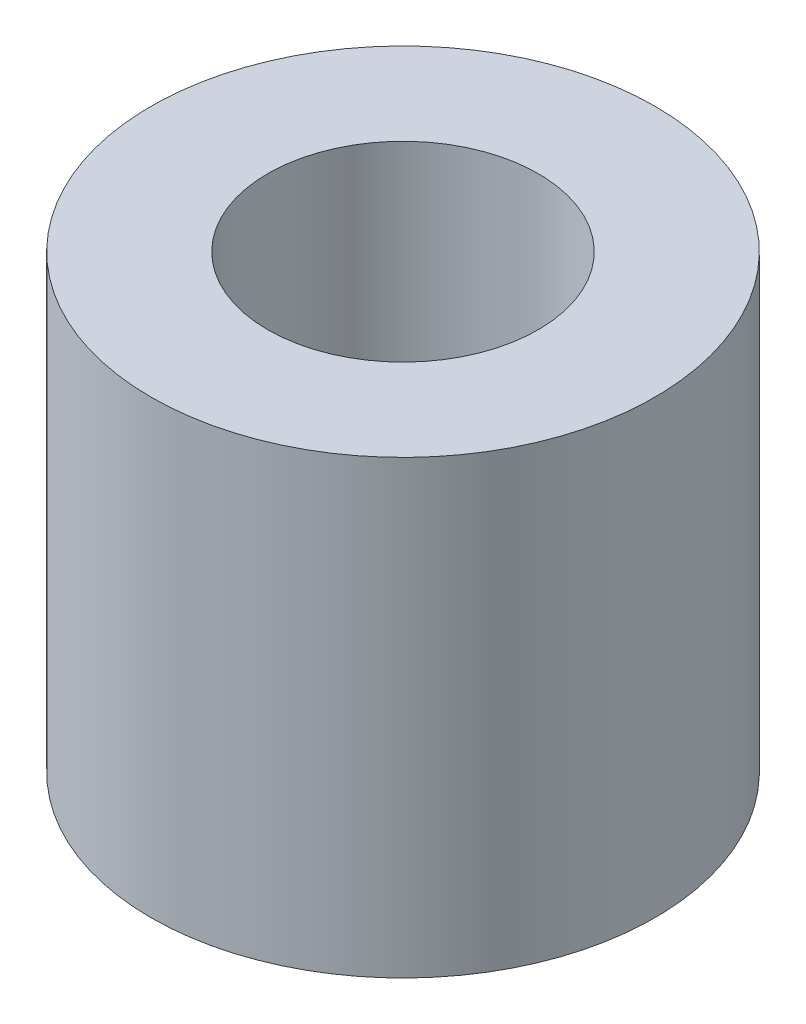
SolidWorks part; units mm, degrees
material "SS400P"
ref_plane "Front Plane" through (0, 0, 0) normal (0, 0, 1) x (1, 0, 0)
ref_plane "Top Plane" through (0, 0, 0) normal (0, 1, 0) x (1, 0, 0)
ref_plane "Right Plane" through (0, 0, 0) normal (1, 0, 0) x (0, 0, -1)
sketch "Sketch1" plane through (0, 0, 0) normal (0, 1, 0) x (1, 0, 0)
  circle A0 centre (0, 0) radius 9.5
  circle A1 centre (0, 0) radius 4.5
  dimension "D1" = 19
  dimension "D2" = 9
extrude "Boss-Extrude1" add sketch "Sketch1" along normal blind 17
hole_wizard "M12 Tapped Hole1" positions "Sketch2" profile "Sketch3" tap size "M12" standard "GB"
sketch "Sketch2" plane through (0, 17, 0) normal (0, 1, 0) x (1, 0, 0)
  point P0 (0, 0)
sketch "Sketch3" plane through (0, 17, 0) normal (1, 0, 0) x (0, 0, 1)
  line L0 (0, 0) -> (0, 35.8144)
  line L1 (0, 35.8144) -> (5.1, 32.75)
  line L2 (5.1, 32.75) -> (5.1, 0)
  line L5 (5.1, 0) -> (0, 0)
  line L10 (0, 35.8144) -> (-5.1, 32.75) construction
  line L11 (0, -6.35) -> (0, 107.95) construction
  dimension "螺纹孔钻头直径" = 10.2
  dimension "螺纹孔钻头深度" = 32.75
  dimension "导头角度" = 118
cosmetic thread "CosmeticThread1"
